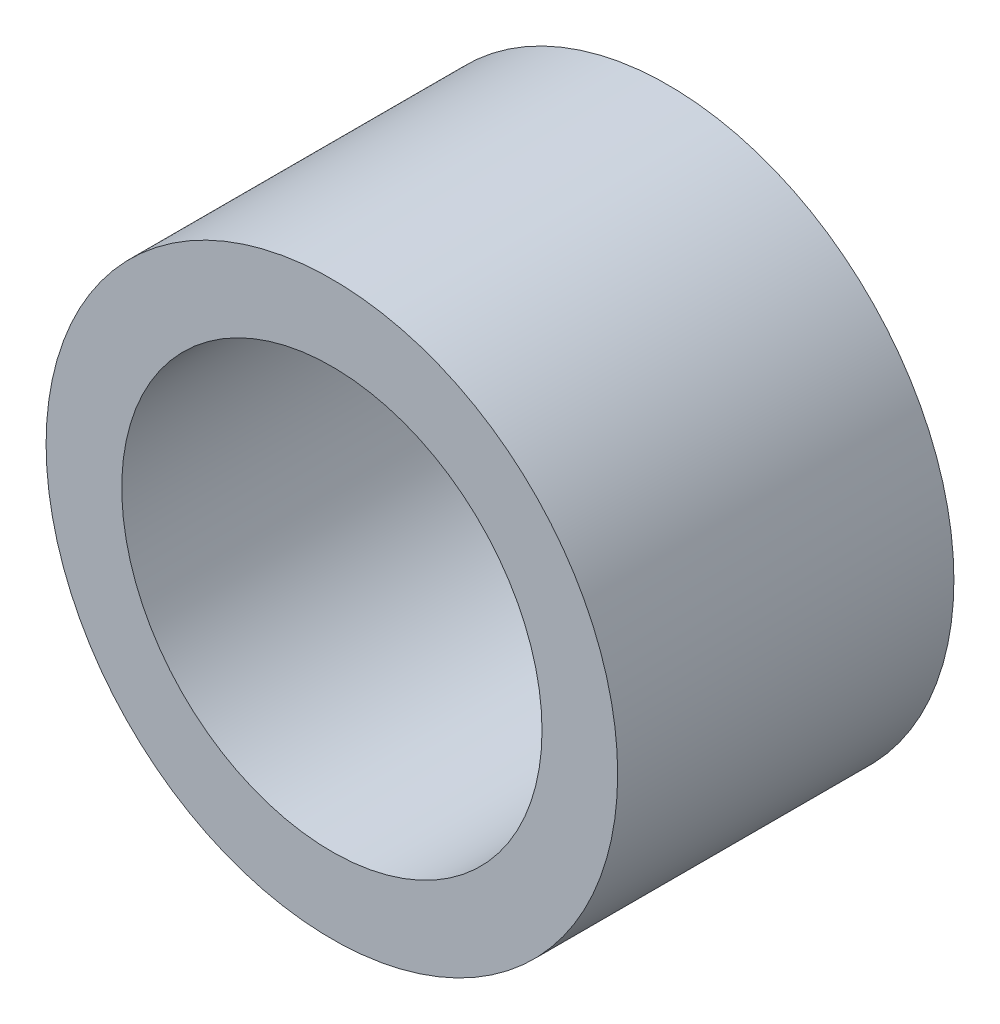
from build123d import *

# Parameters (mm, degrees)
SKETCH_1_R      = 8.5
SKETCH_1_R_2    = 6.25
EXTRUDE_1_DEPTH = 10


with BuildPart() as part:
    # 草图1 → 凸台-拉伸1 (new body)
    with BuildSketch(Plane.XY):
        Circle(SKETCH_1_R)
        Circle(SKETCH_1_R_2, mode=Mode.SUBTRACT)
    extrude(amount=EXTRUDE_1_DEPTH)


solid = part.part
